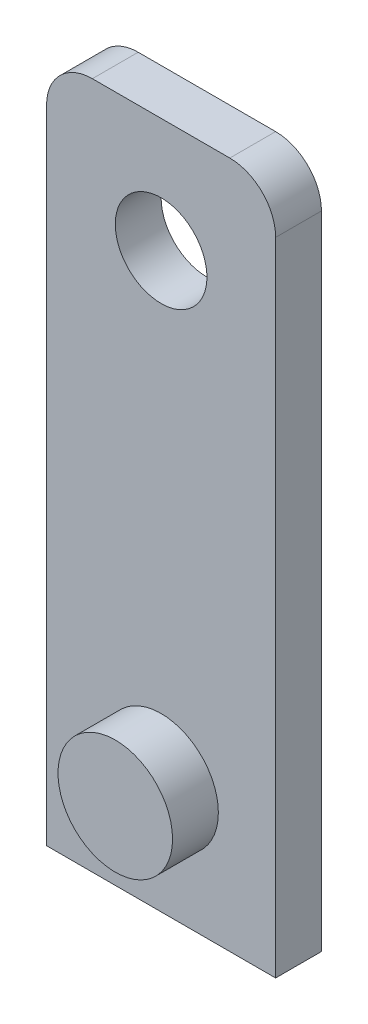
from build123d import *

# Parameters (mm, degrees)
SKETCH_1_R      = 25
EXTRUDE_1_DEPTH = 20
SKETCH_2_W      = 100
SKETCH_2_H      = 300
SKETCH_2_R      = 20
EXTRUDE_2_DEPTH = 20
FILLET_1_R      = 20


with BuildPart() as part:
    # 草图1 → 凸台-拉伸1 (new body)
    with BuildSketch(Plane.XY):
        Circle(SKETCH_1_R)
    extrude(amount=EXTRUDE_1_DEPTH)

    # 草图2 → 凸台-拉伸2 (add)
    with BuildSketch(Plane(origin=(0, 0, 0), x_dir=(-1, 0, 0), z_dir=(0, 0, -1))):
        with Locations((0, 100)):
            Rectangle(SKETCH_2_W, SKETCH_2_H)
        with Locations((0, 200)):
            Circle(SKETCH_2_R, mode=Mode.SUBTRACT)
    extrude(amount=EXTRUDE_2_DEPTH)

    # 圆角1
    fillet_1_edges = [part.edges().sort_by_distance(p)[0] for p in [
        (-50, 250, -10),
        (50, 250, -10),
    ]]
    fillet(fillet_1_edges, radius=FILLET_1_R)


solid = part.part
